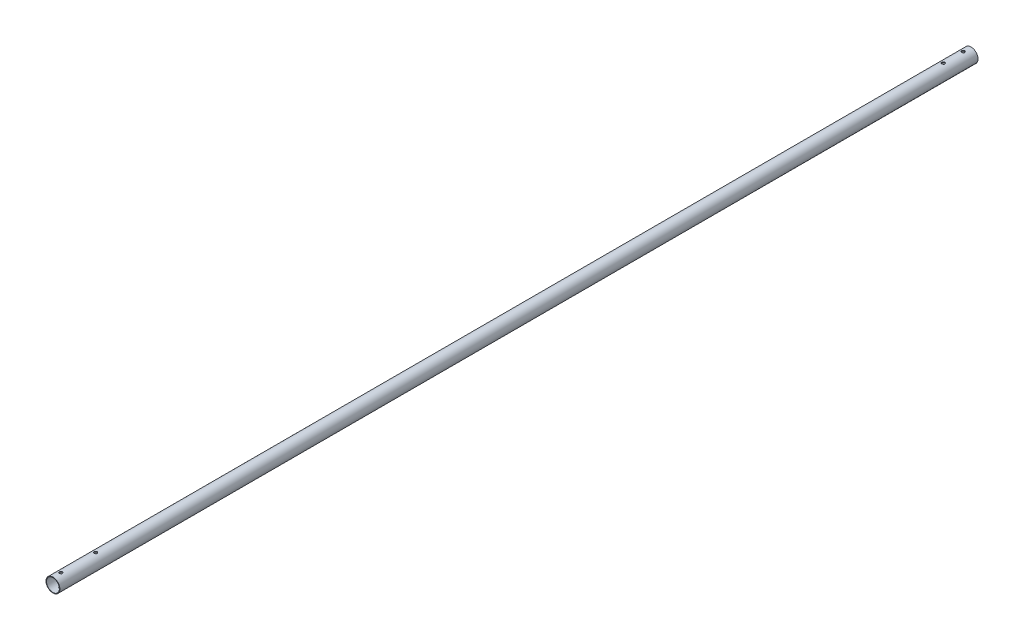
from build123d import *

# Parameters (mm, degrees)
SKETCH_1_R               = 7
SKETCH_1_R_2             = 6.5
EXTRUDE_1_DEPTH          = 926.63
CUT_EXTRUDE_1_DEPTH      = 927.682878281
CUT_EXTRUDE_1_DEPTH_BACK = 927.682878281
SKETCH_2_R               = 1.55


with BuildPart() as part:
    # 草图1 → 凸台-拉伸1 (new body)
    with BuildSketch(Plane.XY):
        Circle(SKETCH_1_R)
        Circle(SKETCH_1_R_2, mode=Mode.SUBTRACT)
    extrude(amount=-EXTRUDE_1_DEPTH)

    # 草图2 → 切除-拉伸1 (cut, two sides: drawn at the far end of the back side and taken through both)
    with BuildSketch(Plane(origin=(0, 0, 0), x_dir=(1, 0, 0), z_dir=(0, 1, 0)).offset(-CUT_EXTRUDE_1_DEPTH_BACK)):
        with Locations(Location((0, 8, 0), (0, 0, 270))):
            Circle(SKETCH_2_R)
        with Locations(Location((0, 43, 0), (0, 0, 270))):
            Circle(SKETCH_2_R)
        with Locations(Location((0, 918.63, 0), (0, 0, 270))):
            Circle(SKETCH_2_R)
        with Locations(Location((0, 898.63, 0), (0, 0, 270))):
            Circle(SKETCH_2_R)
    extrude(amount=CUT_EXTRUDE_1_DEPTH + CUT_EXTRUDE_1_DEPTH_BACK, mode=Mode.SUBTRACT)


solid = part.part
